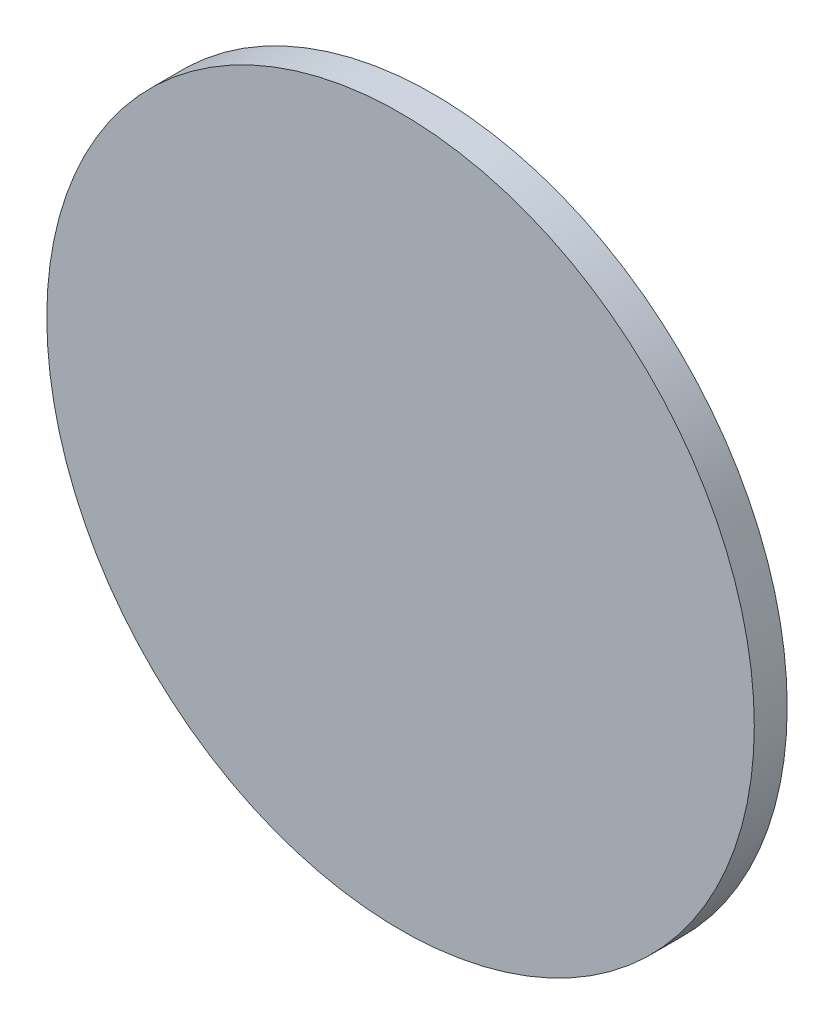
SolidWorks part; units mm, degrees
material "普通碳钢"
ref_plane "Front Plane" through (0, 0, 0) normal (0, 0, 1) x (1, 0, 0)
ref_plane "Top Plane" through (0, 0, 0) normal (0, 1, 0) x (1, 0, 0)
ref_plane "Right Plane" through (0, 0, 0) normal (1, 0, 0) x (0, 0, -1)
sketch "Sketch1" plane through (0, 0, 0) normal (0, 0, 1) x (1, 0, 0)
  circle A0 centre (0, 0) radius 215
  dimension "D1" = 430
extrude "Boss-Extrude1" add sketch "Sketch1" along normal blind 20
